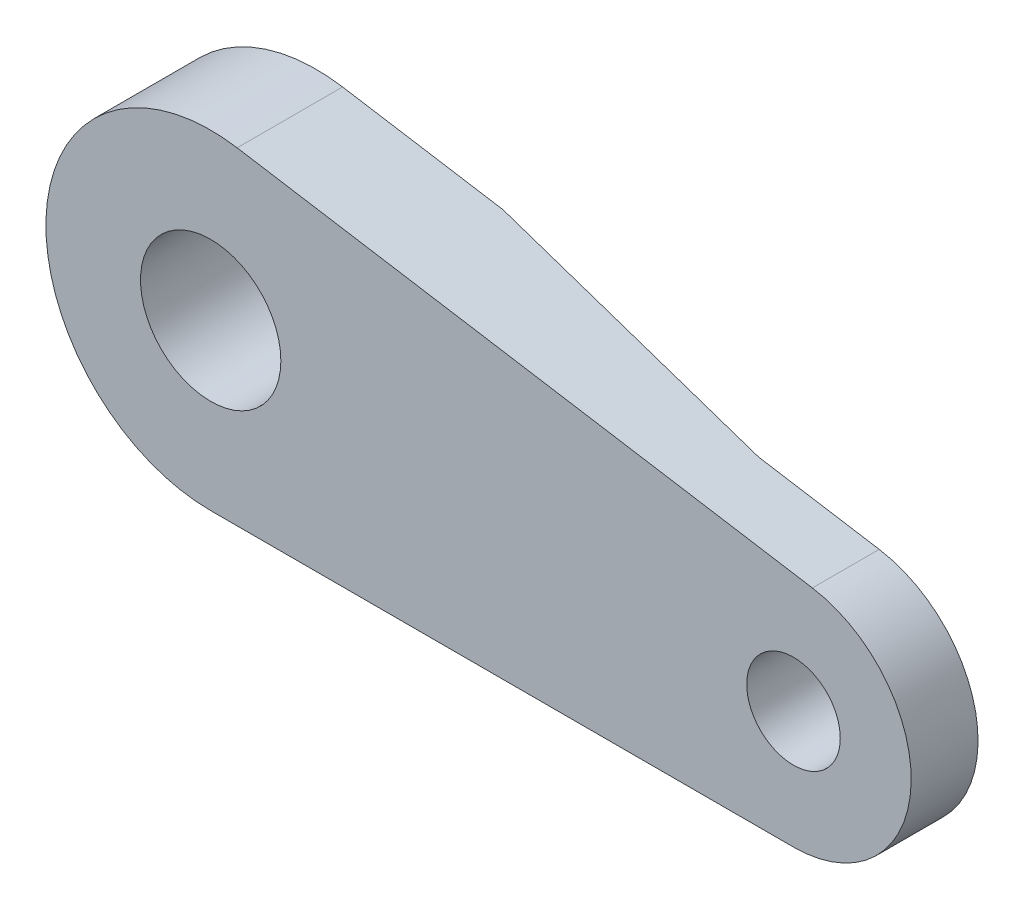
SolidWorks part; units mm, degrees
ref_plane "Front Plane" through (0, 0, 0) normal (0, 0, 1) x (1, 0, 0)
ref_plane "Top Plane" through (0, 0, 0) normal (0, 1, 0) x (1, 0, 0)
ref_plane "Right Plane" through (0, 0, 0) normal (1, 0, 0) x (0, 0, -1)
sketch "Sketch1" plane through (0, 0, 0) normal (0, 0, 1) x (1, 0, 0)
  line L0 (-7.9936, -0.7875) -> (16.9253, -0.7875)
  line L1 (-6.8626, 13.2125) -> (17.7331, 9.2125)
  arc A0 (-6.8626, 13.2125) -> (-7.9936, -0.7875) centre (-7.9936, 6.2582) ccw
  arc A1 (17.7331, 9.2125) -> (16.9253, -0.7875) centre (16.9253, 4.2452) cw
  circle A2 centre (16.9253, 4.2452) radius 2
  circle A3 centre (-7.9936, 6.2582) radius 3
  dimension "D1" = 4
  dimension "D5" = 6
  dimension "D2" = 10
  dimension "D3" = 25
  dimension "D4" = 14
extrude "Boss-Extrude1" add sketch "Sketch1" along normal blind 6
sketch "Sketch2" plane through (0, 0, 0) normal (0, 1, 0) x (1, 0, 0)
  line L0 (29.3866, -3.1416) -> (12.5811, -3.1416)
  line L2 (12.5811, -3.1416) -> (0, -1.4917)
  line L6 (0, -1.4917) -> (-17.0191, -1.4917)
  line L7 (-17.0191, -1.4917) -> (-15.4788, 10.2543)
  line L10 (-15.4788, 10.2543) -> (32.0178, 8.2602)
  line L11 (32.0178, 8.2602) -> (29.3866, -3.1416)
extrude "Cut-Extrude1" cut sketch "Sketch2" against normal through all and the other way through all
sketch "Sketch3" plane through (0, 0, 6) normal (0, 0, 1) x (1, 0, 0)
  point P0 (-7.9936, 6.2582)
  point P1 (16.9253, 4.2452)
